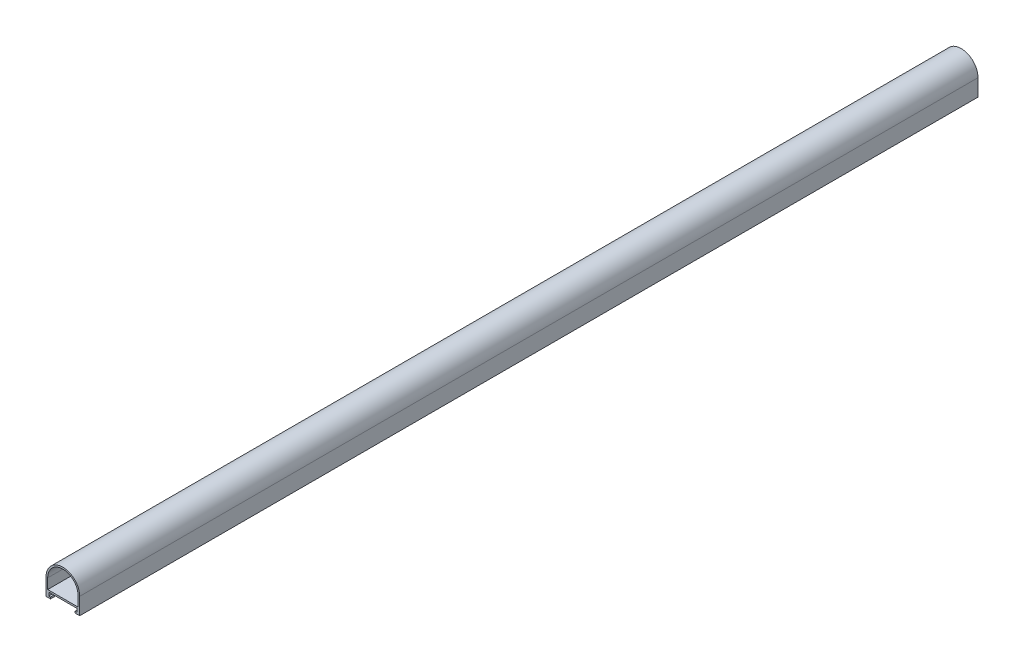
SolidWorks part; units mm, degrees
ref_plane "Front Plane" through (0, 0, 0) normal (0, 0, 1) x (1, 0, 0)
ref_plane "Top Plane" through (0, 0, 0) normal (0, 1, 0) x (1, 0, 0)
ref_plane "Right Plane" through (0, 0, 0) normal (1, 0, 0) x (0, 0, -1)
other "Configuration Table"
sketch "Sketch1" plane through (0, 0, 0) normal (0, 0, 1) x (1, 0, 0)
  line L1 (-25.7644, 0) -> (-25.7644, -15)
  line L2 (-25.7644, -15) -> (-55.7644, -15)
  line L3 (-55.7644, -15) -> (-55.7644, 0)
  arc A0 (-25.7644, 0) -> (-55.7644, 0) centre (-40.7644, 0) ccw
extrude "Boss-Extrude1" add sketch "Sketch1" along normal blind 800
sketch "Sketch2" plane through (0, 0, 800) normal (0, 0, 1) x (1, 0, 0)
  line L0 (-40.7644, 0) -> (-40.7644, -9) construction
  line L1 (-40.7644, -9) -> (-25.7644, -9) construction
  line L2 (-25.7644, -15) -> (-25.7644, 0) construction
  line L3 (-25.7644, -9) -> (-55.7644, -9) construction
  line L4 (-55.7644, 0) -> (-55.7644, -15) construction
  line L5 (-27.2644, 0) -> (-27.2644, -9)
  line L6 (-54.2644, 0) -> (-54.2644, -9)
  line L7 (-54.2644, -9) -> (-27.2644, -9)
  arc A0 (-27.2644, 0) -> (-54.2644, 0) centre (-40.7644, 0) ccw
  arc A1 (-25.7644, 0) -> (-55.7644, 0) centre (-40.7644, 0) ccw construction
  dimension "D1" = 1.5
extrude "Cut-Extrude1" cut sketch "Sketch2" against normal blind 800
sketch "Sketch3" plane through (0, 0, 800) normal (0, 0, 1) x (1, 0, 0)
  line L0 (-55.7644, -15) -> (-51.7644, -15) construction
  line L1 (-55.7644, -15) -> (-25.7644, -15) construction
  line L2 (-51.7644, -15) -> (-51.7644, -13.5)
  line L3 (-51.7644, -13.5) -> (-53.2644, -13.5)
  line L4 (-53.2644, -13.5) -> (-53.2644, -10.5)
  line L5 (-25.7644, -15) -> (-29.7644, -15) construction
  line L6 (-29.7644, -15) -> (-29.7644, -13.5)
  line L7 (-29.7644, -13.5) -> (-28.2644, -13.5)
  line L8 (-28.2644, -13.5) -> (-28.2644, -10.5)
  line L9 (-28.2644, -10.5) -> (-53.2644, -10.5)
  line L10 (-51.7644, -15) -> (-29.7644, -15)
extrude "Cut-Extrude2" cut sketch "Sketch3" against normal through all
